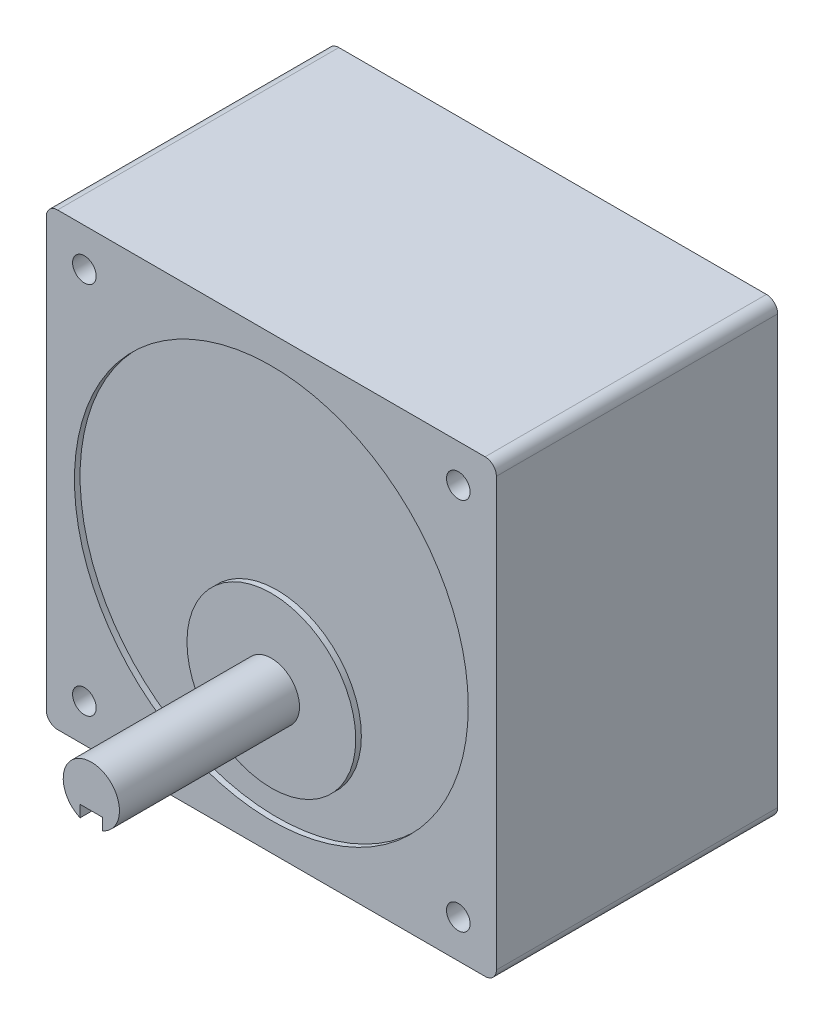
SolidWorks part; units mm, degrees
ref_plane "前视基准面" through (0, 0, 0) normal (0, 0, 1) x (1, 0, 0)
ref_plane "上视基准面" through (0, 0, 0) normal (0, 1, 0) x (1, 0, 0)
ref_plane "右视基准面" through (0, 0, 0) normal (1, 0, 0) x (0, 0, -1)
sketch "草图1" plane through (0, 0, 0) normal (0, 0, 1) x (1, 0, 0)
  line L1 (0, 0) -> (80, 0)
  line L2 (0, 0) -> (0, 80)
  line L3 (0, 80) -> (80, 80)
  line L4 (80, 0) -> (80, 80)
  dimension "D1" = 80
  dimension "D2" = 80
extrude "凸台-拉伸1" add sketch "草图1" along normal blind 50
sketch "草图2" plane through (0, 0, 50) normal (0, 0, 1) x (1, 0, 0)
  line L0 (0, 80) -> (0, 0) construction
  line L1 (80, 80) -> (0, 80) construction
  circle A0 centre (40, 40) radius 35
  dimension "D1" = 40
  dimension "D2" = 70
  dimension "D3" = 40
extrude "切除-拉伸1" cut sketch "草图2" against normal blind 1
fillet "圆角1" radius 2 4 edges at (80, 0, 25) (80, 80, 25) (0, 80, 25) (0, 0, 25)
sketch "草图8" plane through (0, 0, 0) normal (0, 0, -1) x (-1, 0, 0)
  line L0 (-78, 78) -> (-73.234, 73.234) construction
  line L1 (-2, 78) -> (-6.766, 73.234) construction
  line L2 (-6.766, 6.766) -> (-2, 2) construction
  line L3 (-73.234, 6.766) -> (-78, 2) construction
hole_wizard "M5 螺纹孔1" positions "3D草图1" profile "草图9" tap size "M5" standard "Iso" end condition through all
sketch3d "3D草图1"
  point P0 (73.234, 73.234, 0)
  point P3 (6.766, 73.234, 0)
  point P6 (6.766, 6.766, 0)
  point P9 (73.234, 6.766, 0)
sketch "草图9" plane through (73.234, 73.234, 0) normal (1, 0, 0) x (0, 1, 0)
  line L0 (0, 0) -> (0, 50)
  line L1 (0, 50) -> (2.1, 50)
  line L2 (2.1, 50) -> (2.1, 0)
  line L5 (2.1, 0) -> (0, 0)
  line L11 (0, -6.35) -> (0, 107.95) construction
  dimension "通孔螺纹孔钻头直径" = 4.2
  dimension "通孔螺纹孔钻头深度" = 50
cosmetic thread "孔螺蚊线1" parameters "D2"=5
cosmetic thread "孔螺蚊线2" parameters "D2"=5
cosmetic thread "孔螺蚊线3" parameters "D2"=5
cosmetic thread "孔螺蚊线4" parameters "D2"=5
sketch "草图10" plane through (0, 0, 0) normal (0, 0, -1) x (-1, 0, 0)
  circle A0 centre (-40, 40) radius 5
extrude "切除-拉伸2" cut sketch "草图10" against normal blind 20
sketch "草图11" plane through (0, 0, 50) normal (0, 0, 1) x (1, 0, 0)
  line L0 (2, 0) -> (78, 0) construction
  line L1 (0, 78) -> (0, 2) construction
  circle A0 centre (40, 25) radius 5
  dimension "D1" = 10
  dimension "D2" = 25
  dimension "D3" = 40
extrude "凸台-拉伸3" add sketch "草图11" along normal blind 32
sketch "草图13" plane through (0, 0, 82) normal (0, 0, 1) x (1, 0, 0)
  line L1 (42, 22.5) -> (38, 22.5)
  line L2 (42, 22.5) -> (42, 17.5)
  line L3 (42, 17.5) -> (38, 17.5)
  line L4 (38, 22.5) -> (38, 17.5)
  line L5 (42, 22.5) -> (38, 17.5) construction
  line L6 (42, 17.5) -> (38, 22.5) construction
  circle A0 centre (40, 25) radius 5 construction
  point P0 (40, 20)
  dimension "D1" = 5
  dimension "D2" = 4
extrude "切除-拉伸4" cut sketch "草图13" against normal blind 25
sketch "草图14" plane through (0, 0, 49) normal (0, 0, 1) x (1, 0, 0)
  circle A0 centre (40, 25) radius 15
  dimension "D1" = 30
extrude "凸台-拉伸4" add sketch "草图14" along normal blind 1
